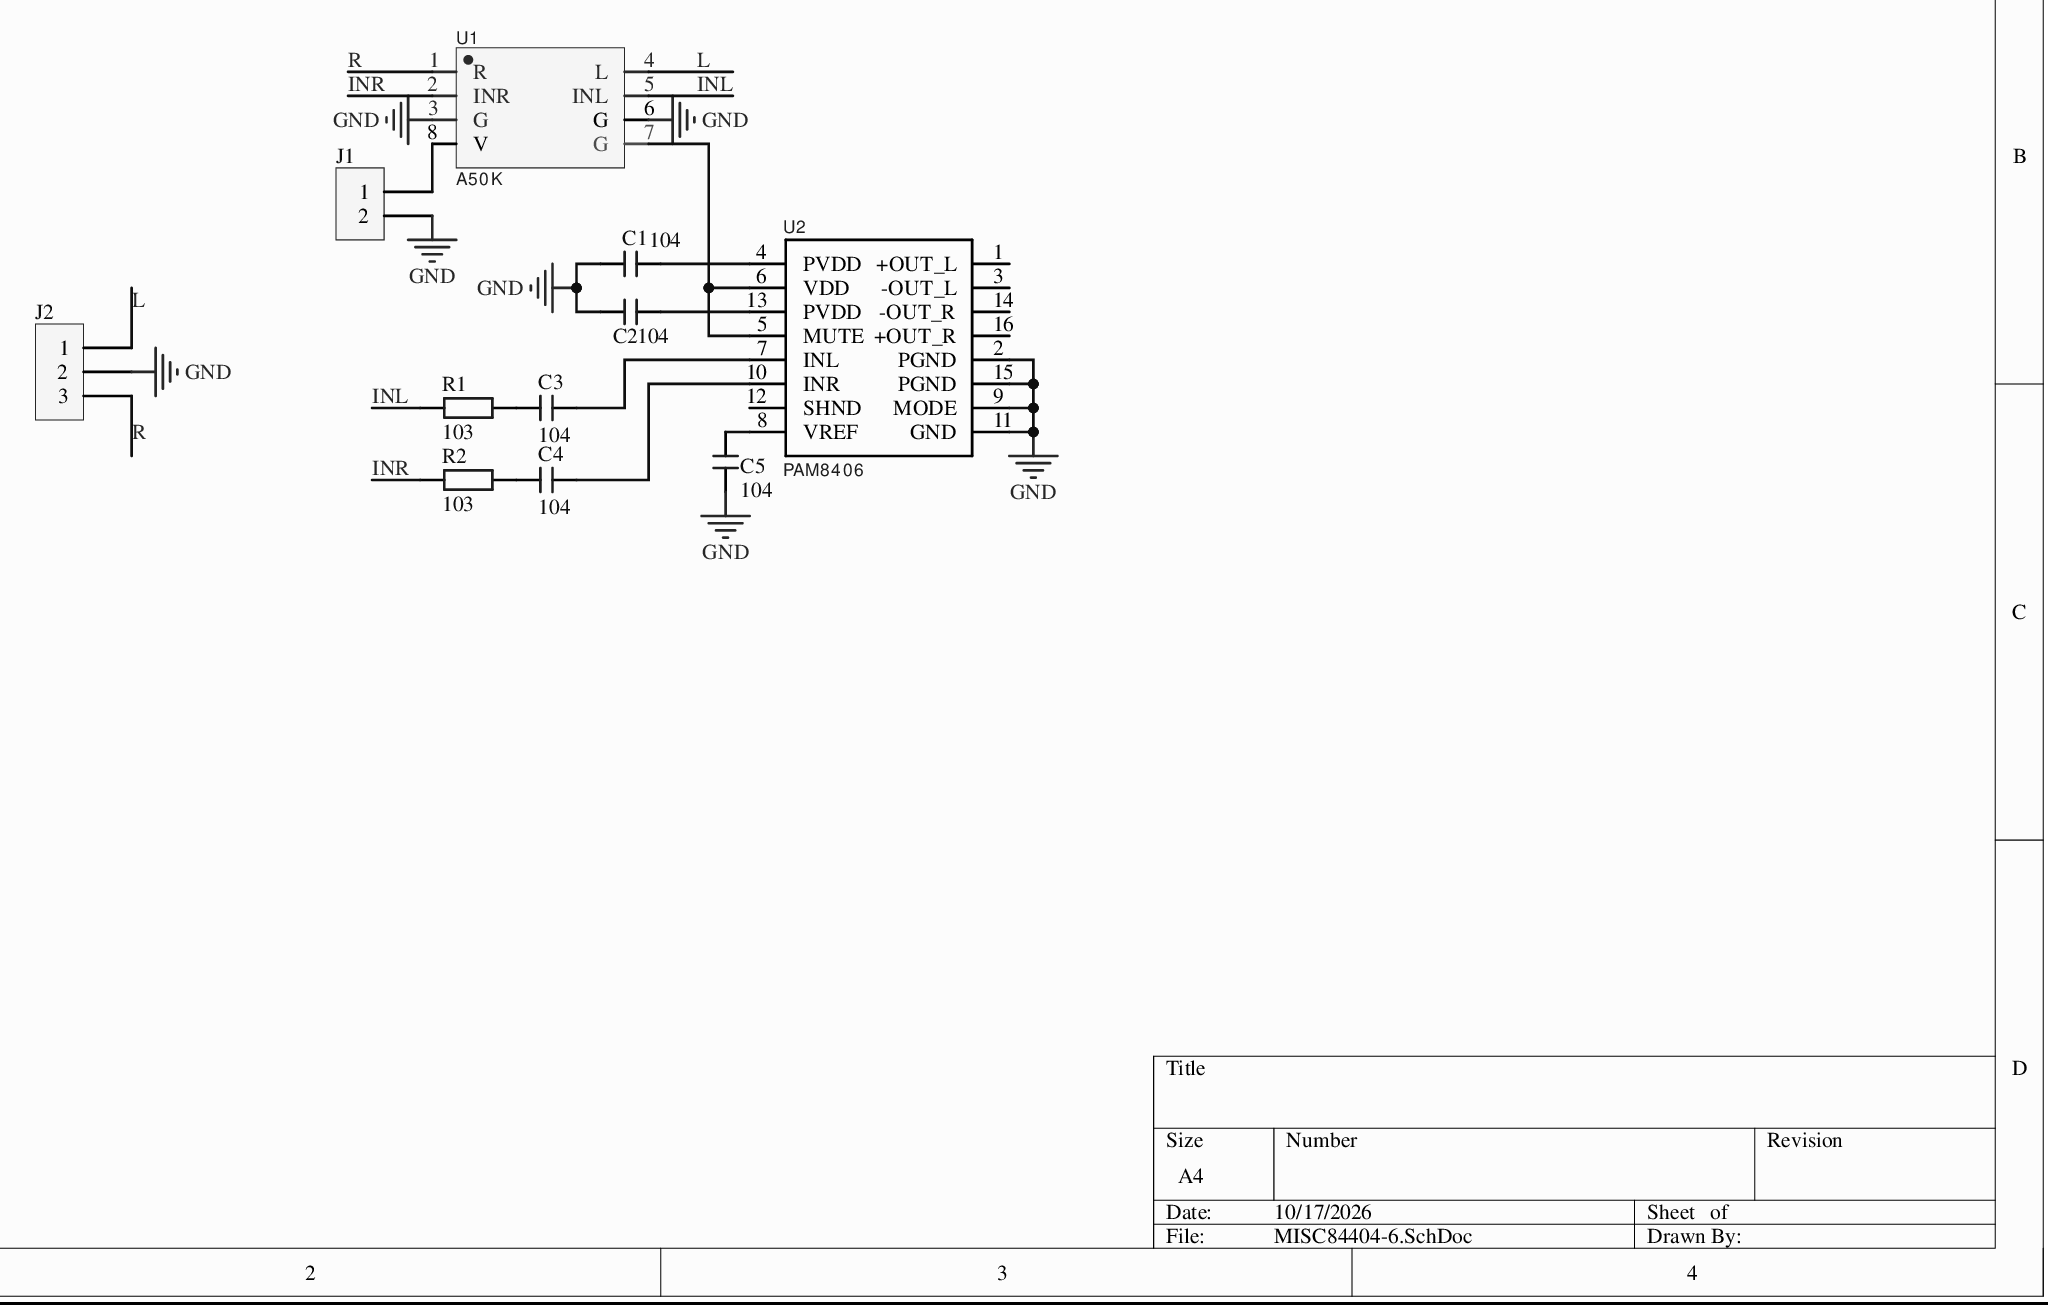
[diagram p0: MISC84404-6.SchDoc]
# Altium project MISC84404-2.PrjPcb
1 sheet, 11 parts. Net scope: global (net labels, ports and power ports of the same name join across sheets).
Board file: MISC84404.PcbDoc

## Sheet MISC84404-6.SchDoc
size A4

### Parts
C1  104  [C 0805_L]
C2  104  [C 0805_L]
C3  104  [C 0805_L]
C4  104  [C 0805_L]
C5  104  [C 0805_L]
J1  Female HDR1X2  [Fe-HDR1X2/2.54-S]  (value not drawn)
J2  Female HDR1X3  [Fe-HDR1X3/2.54-S]  (value not drawn)
R1  103  [R 0805_L]
R2  103  [R 0805_L]
U1  A50K  [SOP-8_L7.0-W7.0-P1.27-LS8.6-BL]
U2  PAM8406  [SOP16]

### Nets
GND: C1.1 C2.1 C5.1 J1.2 J2.2 U1.3(G) U1.6(G) U2.2(PGND) U2.9(MODE) U2.11(GND) U2.15(PGND)
INL: R1.1 U1.5(INL)
INR: R2.1 U1.2(INR)
L: J2.1 U1.4(L)
R: J2.3 U1.1(R)
NetC1_2: C1.2 U2.4(PVDD)
NetC2_2: C2.2 U2.13(PVDD)
NetC3_1: C3.1 U2.7(INL)
NetC3_2: C3.2 R1.2
NetC4_1: C4.1 U2.10(INR)
NetC4_2: C4.2 R2.2
NetC5_2: C5.2 U2.8(VREF)
NetJ1_1: J1.1 U1.8(V)
NetU1_7: U1.7(G) U2.5(MUTE) U2.6(VDD)

Not connected (* = marked no-connect by the designer): U2 1(+OUT_L) 3(-OUT_L) 12(SHND) 14(-OUT_R) 16(+OUT_R)

### Library data of the parts
C1-C5 = C: Chip capacitor; BOM名称: Non-polar chip capacitor
R1 R2 = R: Chip resistor; BOM名称: Chip resistor
U1 = GZP6832A010115KPA50KL